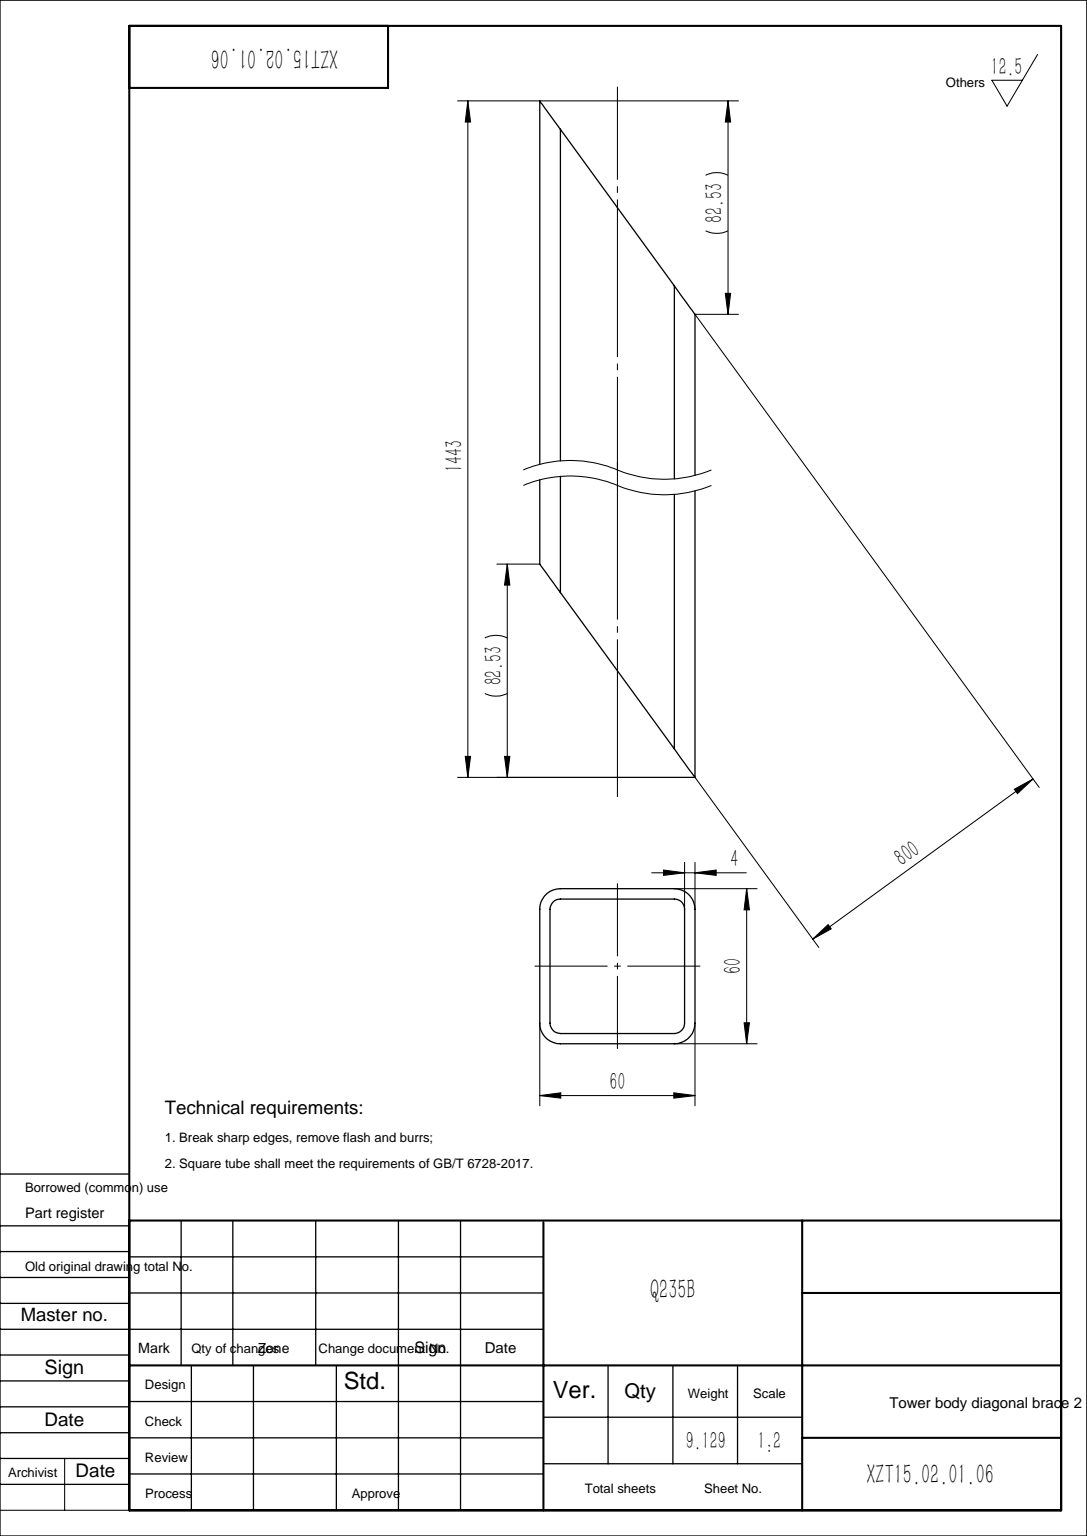
SolidWorks part; units mm, degrees
material "Q235B"
ref_plane "Front Plane" through (0, 0, 0) normal (0, 0, 1) x (1, 0, 0)
ref_plane "Top Plane" through (0, 0, 0) normal (0, 1, 0) x (1, 0, 0)
ref_plane "Right Plane" through (0, 0, 0) normal (1, 0, 0) x (0, 0, -1)
sketch "草图1" plane through (0, 0, 0) normal (0, 0, 1) x (1, 0, 0)
  line L0 (0, 0) -> (0, 1443)
  dimension "D1" = 1443
other "GB/T 6728-2002 square hollow section 60×60×4(1)"
ref_plane "Plane1" through (0, 0, 0) normal (0, 1, 0) x (-1, 0, 0)
sketch "Sketch1" plane through (0, 0, 0) normal (0, 1, 0) x (-1, 0, 0)
  line L0 (-22, -26) -> (22, -26)
  line L1 (-26, -22) -> (-26, 22)
  line L2 (22, 26) -> (-22, 26)
  line L3 (26, 22) -> (26, -22)
  line L4 (-22, -30) -> (22, -30)
  line L5 (-30, -22) -> (-30, 22)
  line L6 (22, 30) -> (-22, 30)
  line L7 (30, 22) -> (30, -22)
  arc A0 (30, 22) -> (22, 30) centre (22, 22) ccw
  arc A1 (22, -30) -> (30, -22) centre (22, -22) ccw
  arc A2 (-30, -22) -> (-22, -30) centre (-22, -22) ccw
  arc A3 (-22, 30) -> (-30, 22) centre (-22, 22) ccw
  arc A4 (-22, 26) -> (-26, 22) centre (-22, 22) ccw
  arc A5 (26, 22) -> (22, 26) centre (22, 22) ccw
  arc A6 (22, -26) -> (26, -22) centre (22, -22) ccw
  arc A7 (-26, -22) -> (-22, -26) centre (-22, -22) ccw
  point P0 (-30, 0)
  point P1 (30, 0)
  point P2 (0, 30)
  point P3 (0, -30)
  point P4 (0, 0)
  point P5 (-30, -30)
  point P6 (30, -30)
  point P7 (30, 30)
  point P8 (-30, 30)
  point P33 (0, 0)
  dimension "D1" = 8
  dimension "Thickness" = 4
  dimension "V_leg" = 60
sketch "Sketch2" plane through (0, 0, 30) normal (0, 0, 1) x (1, 0, 0)
  line L0 (-30, 1443) -> (30, 1360.47)
  line L1 (30, 1443) -> (30, 0) construction
  line L2 (30, 1360.47) -> (30, 1443)
  line L3 (30, 1443) -> (-30, 1443)
  line L4 (-30, 0) -> (-30, 82.53)
  line L5 (-30, 1443) -> (-30, 0) construction
  line L6 (-30, 82.53) -> (30, 0)
  line L7 (30, 0) -> (-30, 0)
  dimension "D1" = 800
  dimension "D2" = 82.53
extrude "Cut-Extrude1" cut sketch "Sketch2" against normal through all both and the other way through all
